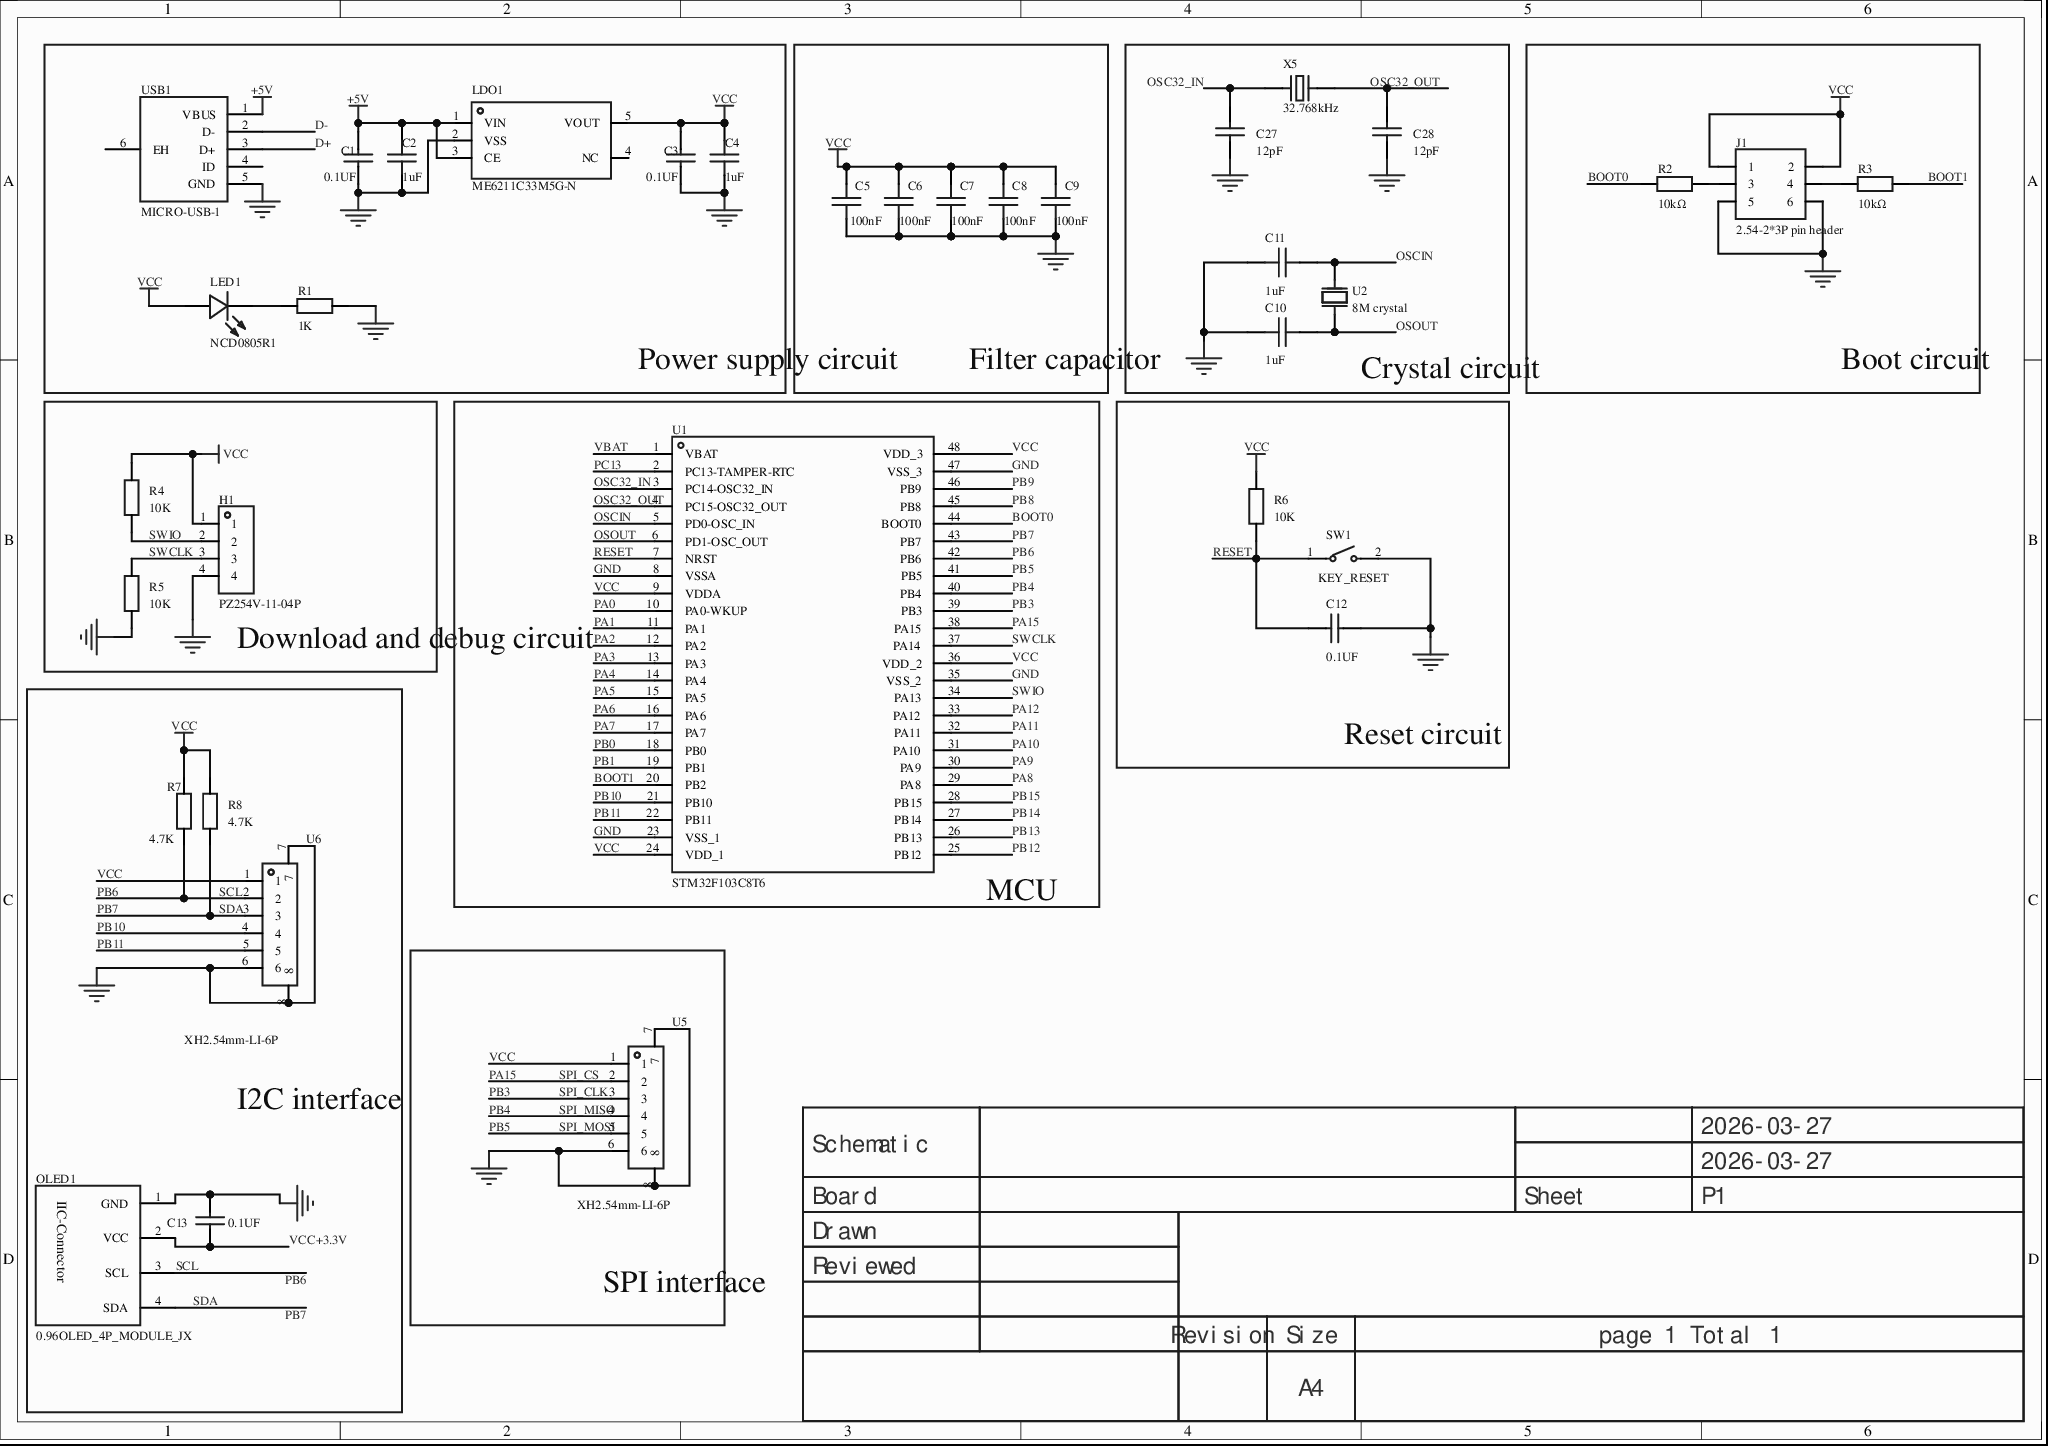
[diagram p0: MISC62287-3.schdoc]
# Altium project MISC62287-2.PrjPcb
1 sheet, 35 parts. Net scope: global (net labels, ports and power ports of the same name join across sheets).
Board file: MISC62287.pcbdoc

## Sheet MISC62287-3.schdoc
size 297 x 209 mm; Version: V1.0; @Project Name: MISC62287; @Update Date: 2026-03-27; @Create Date: 2026-03-27; @Board Name: MISC62287; @Create Time: 22:33:02; @Page Count: 1; @Page No: 1; @Schematic Name: MISC62287; @Update Time: 22:33:02; Size: A4

### Parts
C1  0.1UF  [C0603]
C2  1uF  [C0603]
C3  0.1UF  [C0603]
C4  1uF  [C0603]
C5  100nF  [C0603]
C6  100nF  [C0603]
C7  100nF  [C0603]
C8  100nF  [C0603]
C9  100nF  [C0603]
C10  1uF  [C0603]
C11  1uF  [C0603]
C12  0.1UF  [C0603]
C13  0.1UF  [C0603]
C27  12pF  [R0402]
C28  12pF  [R0402]
H1  PZ254V-11-04P  [HDR-TH_4P-P2.54-V-M]
J1  2.54-2*3P pin header  [HDR-TH_6P-P2.54-V-M-R2-C3-S2.54-1]
LDO1  ME6211C33M5G-N  [SOT-23-5_L3.0-W1.7-P0.95-LS2.8-BL]
LED1  NCD0805R1  [LED0805-RD]
OLED1  0.96OLED_4P_MODULE_JX  [0.96OLED_4P]
R1  1K  [R0603]
R2  10kΩ  [R0603]
R3  10kΩ  [R0603]
R4  10K  [R0603]
R5  10K  [R0603]
R6  10K  [R0603]
R7  4.7K  [R0603]
R8  4.7K  [R0603]
SW1  KEY_RESET  [SW-SMD_L6.0-W3.3-LS8.0]
U1  STM32F103C8T6  [LQFP-48_L7.0-W7.0-P0.50-LS9.0-BL]
U2  8M crystal  [HC-49S_L11.5-W4.7-P4.88]
U5  XH2.54mm-LI-6P  [CONN-SMD_6P-P2.50-H]
U6  XH2.54mm-LI-6P  [CONN-SMD_6P-P2.50-H]
USB1  MICRO-USB-1  [MICRO-USB-SMD_C9900008946]
X5  32.768kHz  [OSC-SMD_L3.2-W1.5]

### Blocks framed on the sheet
Power supply circuit: C1-C4 LDO1 LED1 R1 USB1
Filter capacitor: C5-C9
Crystal circuit: C10 C11 C27 C28 U2 X5
Boot circuit: J1 R2 R3
Download and debug circuit: H1 R4 R5
MCU: U1
Reset circuit: C12 R6 SW1
I2C interface: C13 OLED1 R7 R8 U6
SPI interface: U5

### Nets
+5V: C1.2 C2.2 LDO1.1(VIN) LDO1.3(CE) USB1.1(VBUS)
GND: C1.1 C2.1 C3.1 C4.1 C5.1 C6.1 C7.1 C8.1 C9.1 C10.2 C11.2 C12.1 C13.2 C27.1 C28.1 H1.4 J1.5 J1.6 LDO1.2(VSS) OLED1.1(GND) R1.2 R5.1 SW1.2 U1.8(VSSA) U1.23(VSS_1) U1.35(VSS_2) U1.47(VSS_3) U5.6 U5.7 U5.8 U6.6 U6.7 U6.8 USB1.5(GND)
VCC: C3.2 C4.2 C5.2 C6.2 C7.2 C8.2 C9.2 H1.1 J1.1 J1.2 LDO1.5(VOUT) LED1.2(+) R4.2 R6.2 R7.2 R8.2 U1.9(VDDA) U1.24(VDD_1) U1.36(VDD_2) U1.48(VDD_3) U5.1 U6.1
BOOT0: R2.1 U1.44(BOOT0)
BOOT1: R3.2 U1.20(PB2)
D+: USB1.3(D+)
D-: USB1.2(D-)
OSC32_IN: C27.2 U1.3(PC14-OSC32_IN) X5.1
OSC32_OUT: C28.2 U1.4(PC15-OSC32_OUT) X5.2
OSCIN: C11.1 U1.5(PD0-OSC_IN) U2.1(OSC1)
OSOUT: C10.1 U1.6(PD1-OSC_OUT) U2.2(OSC2)
PA0: U1.10(PA0-WKUP)
PA1: U1.11(PA1)
PA2: U1.12(PA2)
PA3: U1.13(PA3)
PA4: U1.14(PA4)
PA5: U1.15(PA5)
PA6: U1.16(PA6)
PA7: U1.17(PA7)
PA8: U1.29(PA8)
PA9: U1.30(PA9)
PA10: U1.31(PA10)
PA11: U1.32(PA11)
PA12: U1.33(PA12)
PA15: U1.38(PA15) U5.2  [also labelled SPI_CS]
PB0: U1.18(PB0)
PB1: U1.19(PB1)
PB3: U1.39(PB3) U5.3  [also labelled SPI_CLK]
PB4: U1.40(PB4) U5.4  [also labelled SPI_MISO]
PB5: U1.41(PB5) U5.5  [also labelled SPI_MOSI]
PB6: OLED1.3(SCL) R7.1 U1.42(PB6) U6.2  [also labelled SCL]
PB7: OLED1.4(SDA) R8.1 U1.43(PB7) U6.3  [also labelled SDA]
PB8: U1.45(PB8)
PB9: U1.46(PB9)
PB10: U1.21(PB10) U6.4
PB11: U1.22(PB11) U6.5
PB12: U1.25(PB12)
PB13: U1.26(PB13)
PB14: U1.27(PB14)
PB15: U1.28(PB15)
PC13: U1.2(PC13-TAMPER-RTC)
RESET: C12.2 R6.1 SW1.1 U1.7(NRST)
SWCLK: H1.3 R5.2 U1.37(PA14)
SWIO: H1.2 R4.1 U1.34(PA13)
VBAT: U1.1(VBAT)
VCC+3.3V: C13.1 OLED1.2(VCC)
NetJ1_3: J1.3 R2.2
NetJ1_4: J1.4 R3.1
NetLED1_1: LED1.1(-) R1.1

Not connected (* = marked no-connect by the designer): LDO1 4(NC)*; USB1 4(ID)* 6(EH)*

### Notes on the sheet
- 2026-03-27
- Schematic
- Board
- Sheet
- P1
- Drawn
- Reviewed
- Revision
- Size
- A4
- page 1 Total 1

### Library data of the parts
C1 C3 C12 = CAPCER0.1UF16VX5R0603,CAPCER0.1UF25VX5R0603,CAPCER0.1UF16VX7R0603: AddInBom: yes; ModelId: ac125912035d415993ca9572d50418b10819f05c4eef4c71ace90d822a990e87; ModelName: C0603_L1.6-W0.8-H0.8; ModelTransform: 62.992,31.496,0,0,0,0,0,0,0; Symbol: CAPCER0.1UF16VX5R0603,CAPCER0.1UF25VX5R0603,CAPCER0.1UF16VX7R0603; Device: CAPCER0.1UF16VX5R0603,CAPCER0.1UF25VX5R0603,CAPCER0.1UF16VX7R0603; Manufacturer Part: 0.1UF; LCSC Part Name: CAPCER0.1UF16VX5R0603,CAPCER0.1UF25VX5R0603,CAPCER0.1UF16VX7R0603; SupplierPart: C9900012833; Supplier Footprint: C0603; JLCPCB Part Class: Extended Part; Supplier: LCSC; ConvertToPcb: yes; FootprintName: C0603
C2 C4 C10 C11 = CL10A105KB8NNNC: Capacitance:1uF;Tolerance:±10%;Rated voltage:50V;Temperature coefficient:X5R;; Manufacturer: SAMSUNG(三星); AddInBom: yes; ModelId: ac125912035d415993ca9572d50418b10819f05c4eef4c71ace90d822a990e87; ModelName: C0603_L1.6-W0.8-H0.8; ModelTransform: 62.992,31.496,0,0,0,0,0,0,0; Tolerance: ±10%; Voltage Rating: 50V; Temperature Coefficient: X5R; Symbol: CL10A105KB8NNNC; Device: CL10A105KB8NNNC; LCSC Part Name: 1uF ±10% 50V; SupplierPart: C15849; ManufacturerPart: CL10A105KB8NNNC; Supplier Footprint: 0603; JLCPCB Part Class: Basic Part; Datasheet: https://example.com/datasheet/16531.html; Supplier: LCSC; ConvertToPcb: yes; FootprintName: C0603; Value: 1uF
C5-C9 = CC0603KPX7R7BB104: Capacitance:100nF;Tolerance:±10%;Rated voltage:16V;Temperature coefficient:X7R;; Manufacturer: YAGEO(国巨); AddInBom: yes; ModelId: ac125912035d415993ca9572d50418b10819f05c4eef4c71ace90d822a990e87; ModelName: C0603_L1.6-W0.8-H0.8; ModelTransform: 62.992,31.496,0,0,0,0,0,0,0; Tolerance: ±10%; Voltage Rating: 16V; Temperature Coefficient: X7R; Symbol: CC0603KPX7R7BB104; Device: CC0603KPX7R7BB104; LCSC Part Name: 100nF ±10% 16V; SupplierPart: C2649559; ManufacturerPart: CC0603KPX7R7BB104; Supplier Footprint: 0603; JLCPCB Part Class: Extended Part; Datasheet: https://example.com/datasheet/2741468.html; Supplier: LCSC; ConvertToPcb: yes; FootprintName: C0603; Value: 100nF
C13 = CAPCER0.1UF16VX5R0603,CAPCER0.1UF25VX5R0603,CAPCER0.1UF16VX7R0603: 3D Model: ac125912035d415993ca9572d50418b10819f05c4eef4c71ace90d822a990e87; 3D Model Transform: 62.992,31.496,0,0,0,0,0,0,0; AddInBom: yes; ModelName: C0603_L1.6-W0.8-H0.8; Symbol: CAPCER0.1UF16VX5R0603,CAPCER0.1UF25VX5R0603,CAPCER0.1UF16VX7R0603; Device: CAPCER0.1UF16VX5R0603,CAPCER0.1UF25VX5R0603,CAPCER0.1UF16VX7R0603; Manufacturer Part: 0.1UF; LCSC Part Name: CAPCER0.1UF16VX5R0603,CAPCER0.1UF25VX5R0603,CAPCER0.1UF16VX7R0603; Supplier Part: C9900012833; Supplier Footprint: C0603; JLCPCB Part Class: Extended Part; Supplier: LCSC; ConvertToPcb: yes; FootprintName: C0603
C27 C28 = 0402CG120J500NT: Capacitance:12pF;Tolerance:±5%;Rated voltage:50V;Material (temperature coefficient):C0G;; Manufacturer: FH(风华); 3D Model: 36a51122f27c49738f86b3bfa98863e0; 3D Model Transform: 39.37,19.685,0,0,0,0,0,0,0; Tolerance: ±5%; Voltage Rated: 50V; Temperature Coefficient: C0G; AddInBom: yes; ModelName: C0402_L1.0-W0.5-H0.5; Symbol: 0402CG120J500NT; Device: 0402CG120J500NT; Value: 12pF; LCSC Part Name: 12pF ±5% 50V; Supplier Part: C1547; Manufacturer Part: 0402CG120J500NT; Supplier Footprint: 0402; JLCPCB Part Class: Basic library; Datasheet: https://example.com/pdf/20200305/C486355_26A10D38EF8C2A5C37091D0039909270.pdf; Supplier: LCSC; ConvertToPcb: yes; FootprintName: R0402
H1 = PZ254V-11-04P: Pin structure:1x4P;Pitch:2.54mm;Row spacing:-;Round/square pin:Square;Mounting:Through-hole;Rows:Single row;Total pin count:4P;Rated current:3A;Rated voltage:250V;Mating pin length:6mm;Plastic height:2.5mm;Terminal pin length:3mm;Contact material:-;Operating temperature:-40℃~+105℃;Color:Black;; Manufacturer: XFCN(兴飞); Symbol: PZ254V-11-04P_C2691448; AddInBom: yes; ModelId: 112f4d05e8d64e99ab9a333894bea4f90819f05c4eef4c71ace90d822a990e87; ModelName: HDR-TH_4P-P2.54-M-LI-1X4P; ModelTransform: 399.999,104.7242,0,0,0,0,0,0,-118.11; Pin Structure: 1x4P; Pitch: 2.54mm; Circluar Pins/Square Pins: Square; Current Rating: 3A; Voltage Rating (Max): 250V; Device: PZ254V-11-04P; LCSC Part Name: 1x4P 间距:2.54mm 方针 直插; SupplierPart: C2691448; ManufacturerPart: PZ254V-11-04P; Supplier Footprint: 插件,P=2.54mm; JLCPCB Part Class: Extended Part; Datasheet: https://example.com/datasheet/PZ254V-11-04P/2801085.html; Supplier: LCSC; ConvertToPcb: yes; FootprintName: HDR-TH_4P-P2.54-V-M; Row Spacing: -; Mounting Type: Through-hole; Number of Rows: Single row; Number of Pins: 4P; Length of Mating Pin: 6mm; Insulation Height: 2.5mm; Length of End Connection Pin: 3mm; Contact Material: -; Operating Temperature: -40℃~+105℃; Color: Black
J1 = 2.54-2*3P针: Pin structure:-;Pitch:2.54mm;Row spacing:2.54mm;Round/square pin:-;Mounting:Through-hole;Rows:Dual row;Total pin count:6P;Rated current:-;Rated voltage:-;Mating pin length:-;Plastic height:-;Contact material:-;Contact plating:-;Color:Black;; Manufacturer: BOOMELE(博穆精密); Symbol: Header-Male-2.54_2x3; AddInBom: yes; ModelId: fd1b55b786fb415ca65c4187088147b70819f05c4eef4c71ace90d822a990e87; ModelName: HDR2.54-M-LI-2x3P; ModelTransform: 299.9994,200,0,0,0,0,0,0,-118.11; Pitch: 2.54mm; Device: 2.54-2*3P pin header; LCSC Part Name: 间距:2.54mm 直插; SupplierPart: C65114; ManufacturerPart: 2.54-2*3P针; Supplier Footprint: 插件,P=2.54mm; JLCPCB Part Class: Extended Part; Supplier: LCSC; ConvertToPcb: yes; FootprintName: HDR-TH_6P-P2.54-V-M-R2-C3-S2.54-1; Pin Structure: -; Row Spacing: 2.54mm; Circluar Pins/Square Pins: -; Mounting Type: Through-hole; Number of Rows: Dual row; Number of Pins: 6P; Current Rating: -; Voltage Rating (Max): -; Length of Mating Pin: -; Insulation Height: -; Contact Material: -; Contact Plating: -; Color: Black
LDO1 = ME6211C33M5G-N: Output type:Fixed;Operating voltage:6V;Output voltage:3.3V;Output current:500mA;PSRR:70dB@(1kHz);Output polarity:Positive;; Manufacturer: MICRONE(南京微盟); AddInBom: yes; ModelId: 0a2a1b8f50944f73965918ad6e5fe1670819f05c4eef4c71ace90d822a990e87; ModelName: SOT-23-5_L2.9-W1.6-H1.1-LS2.8-P0.95; ModelTransform: 118.60433,114.173,0,90,0,0,0.0005,0.0005,0; Output Type: Fixed; Voltage - Supply: 6V; Output Voltage: 3.3V; Output Current: 500mA; Voltage Dropout: 120mV@(100mA); standby current: 60uA; Noise: 50uVrms; Number of Outputs: 1; Symbol: ME6211C33M5G-N; Device: ME6211C33M5G-N; LCSC Part Name: 输入6V 输出3.3V 500mA; SupplierPart: C82942; ManufacturerPart: ME6211C33M5G-N; Supplier Footprint: SOT-23-5; JLCPCB Part Class: Extended Part; Datasheet: https://example.com/datasheet/84106.html; Supplier: LCSC; ConvertToPcb: yes; FootprintName: SOT-23-5_L3.0-W1.7-P0.95-LS2.8-BL; Power Supply Rejection Ratio (PSRR): 70dB@(1kHz); Features: Overcurrent protection; enable; short-circuit protection; Operating Temperature: -40℃~+150℃; Output Configuration: Positive
LED1 = NCD0805R1: Lamp head type:-;Emission color:Red;Forward voltage drop (Vf):1.6V~2.6V;Power:65mW;Forward current:25mA;Wavelength:615nm~630nm;Diode configuration:Discrete diode;Lens color:-;Color temperature:-;Luminous intensity:195mcd;Viewing angle:130°;Packaging:-;Operating temperature:-30℃~+85℃;; Manufacturer: 国星光电; Symbol: FC-2012HRK-620D; AddInBom: yes; ModelId: b1c5ed7a4f6e46d3bc6f6cc7c20f3fea0819f05c4eef4c71ace90d822a990e87; ModelTransform: 79.527,49.2125,0,0,0,0,0,0,0; Illumination Color: Red; Power(Watts): 65mW; Forward Current: 25mA; Peak Wavelength: 630nm; Luminous Intensity: 195mcd; Viewing Angle: 130°; Device: NCD0805R1; LCSC Part Name: 片式发光二极管; SupplierPart: C84256; ManufacturerPart: NCD0805R1; Supplier Footprint: 0805; JLCPCB Part Class: Basic Part; Datasheet: https://example.com/datasheet/85425.html; Supplier: LCSC; ConvertToPcb: yes; FootprintName: LED0805-RD; ModelName: LED0805-RD; Lamp Holder Type: -; Voltage - Forward(Vf): 1.6V~2.6V; Wavelength - Dominant: 615nm~630nm; Diode Configuration: Discrete diode; Lens Color: -; Color Temperature: -; Mounting Style: -; Operating Temperature: -30℃~+85℃
OLED1 = 0.96OLED_4P_MODULE_JX: AddInBom: yes; ModelId: 79c000fdb68d45a296c2e9bedf4f90550819f05c4eef4c71ace90d822a990e87; ModelTransform: 1393.69792,1318.895,0,0,0,0,0,-560.079,-137.795; Symbol: 0.96OLED_4P_MODULE_JX; Device: 0.96OLED_4P_MODULE_JX; LCSC Part Name: 0.96OLED_4P_MODULE_JX; SupplierPart: C9900004566; ManufacturerPart: 0.96OLED_4P_MODULE_JX; Supplier Footprint: 插件; JLCPCB Part Class: Extended Part; Supplier: LCSC; ConvertToPcb: yes; FootprintName: 0.96OLED_4P; ModelName: 0.96OLED_4P
R1 R4-R8 = Res_0603: Symbol: Resistor; ConvertToPcb: yes; ModelId: fc143cca1e79419f9cd78b61e9279f080819f05c4eef4c71ace90d822a990e87; ModelTransform: 31.8897,63.7794,0,90,0,0,0,0,0; Device: Res_0603; AddInBom: yes; Supplier Footprint: 0603; FootprintName: R0603; ModelName: R0603
  R1: Value: 1K
  R4-R6: Value: 10K
  R7 R8: Value: 4.7K
R2 R3 = 0603WAF1002T5E: Resistor type:Thick-film resistor;Resistance:10kΩ;Tolerance:±1%;Power:100mW;Operating voltage:75V;Temperature coefficient:±100ppm/℃;; Manufacturer: UNI-ROYAL(厚声); AddInBom: yes; ModelId: fc143cca1e79419f9cd78b61e9279f080819f05c4eef4c71ace90d822a990e87; ModelTransform: 31.8897,63.7794,0,90,0,0,0,0,0; Tolerance: ±1%; Power(Watts): 100mW; Voltage-Supply(Max): 75V; Symbol: 0603WAF1002T5E; Device: 0603WAF1002T5E; LCSC Part Name: 厚膜电阻 10kΩ ±1% 100mW; SupplierPart: C25804; ManufacturerPart: 0603WAF1002T5E; Supplier Footprint: 0603; JLCPCB Part Class: Basic Part; Datasheet: https://example.com/datasheet/26547.html; Supplier: LCSC; ConvertToPcb: yes; FootprintName: R0603; ModelName: R0603; Type: Thick-film resistor; Value: 10kΩ; Temperature Coefficient: ±100ppm/℃; Operating Temperature: -55℃~+155℃
SW1 = SW_PB2_A1: AddInBom: yes; ModelId: b2f4ea9f0afc4b0786d53dba66ceb9e40819f05c4eef4c71ace90d822a990e87; ModelName: SW-SMD_L6.0-W3.3-H5-LS8.0; ModelTransform: 314.96,129.921,0,0,0,0,0,0,0; Symbol: SW_PB2_A1; Device: SW_PB2_A1; Manufacturer Part: KEY_RESET; LCSC Part Name: SW_PB2_A1; SupplierPart: C9900015236; Supplier Footprint: SW_3*6*2.5mm; JLCPCB Part Class: Extended Part; Supplier: LCSC; ConvertToPcb: yes; FootprintName: SW-SMD_L6.0-W3.3-LS8.0
U1 = STM32F103C8T6: CPU core:ARM-M3;Max CPU frequency:72MHz;Application field:-;; Manufacturer: ST(意法半导体); AddInBom: yes; ModelId: 093be70396ff421eb2cdb946d5311efc0819f05c4eef4c71ace90d822a990e87; ModelName: LQFP-48_L7.0-W7.0-H1.4-LS9.0-P0.50; ModelTransform: 354.331,354.331,0,0,0,0,0,0,0; CPU Core: ARM-M3; CPU Maximum Speed: 72MHz; Program Storage Size: 64KB; Program Memory Type: FLASH; Number of I/O: 37; ADC (Bit): 12bit; Voltage - Supply: 2V~3.6V; Symbol: STM32F103C8T6; Device: STM32F103C8T6; LCSC Part Name: 主流增强型ARM Cortex-M3 MCU，具有64 KB Flash、72 MHz CPU、电机控制、USB和CAN; SupplierPart: C8734; ManufacturerPart: STM32F103C8T6; Supplier Footprint: LQFP-48(7x7); JLCPCB Part Class: Extended Part; Datasheet: https://example.com/datasheet/9243.html; Supplier: LCSC; ConvertToPcb: yes; FootprintName: LQFP-48_L7.0-W7.0-P0.50-LS9.0-BL; Applications: -
U2 = 8M晶振_C9900011272: ManufacturerPart: 8M晶振; Device: 8M crystal_C9900011272; AddInBom: yes; ModelId: 8681f9edbc4c49baa7439b9863851e5c0819f05c4eef4c71ace90d822a990e87; ModelTransform: 452.755,183.4642,0,0,0,0,0,0,-137.795; Symbol: 8M crystal; LCSC Part Name: 8M晶振; SupplierPart: C9900011272; Supplier Footprint: HC-49S; JLCPCB Part Class: Extended Part; Supplier: LCSC; ConvertToPcb: yes; FootprintName: HC-49S_L11.5-W4.7-P4.88; ModelName: HC-49S_L11.5-W4.7-P4.88
U5 U6 = XH2.54mm-LI-6P: AddInBom: yes; ModelId: d00e98fc2787443b99850c08410b29640819f05c4eef4c71ace90d822a990e87; ModelTransform: 787.4,401.574,0,0,0,0,0,-6.89,0; Symbol: XH2.54MM-LI-6P; Device: XH2.54mm-LI-6P; LCSC Part Name: XH2.54mm-LI-6P; SupplierPart: C2842318; ManufacturerPart: XH2.54mm-LI-6P; Supplier Footprint: SMD-6_7.8X17.5X2.5P; JLCPCB Part Class: Extended Part; Supplier: LCSC; ConvertToPcb: yes; FootprintName: CONN-SMD_6P-P2.50-H; ModelName: CONN-SMD_6P-P2.50-H
USB1 = MICRO-USB-1: AddInBom: yes; ModelId: 03278485a0ad4b6f9ea4a64b4dabf4cb0819f05c4eef4c71ace90d822a990e87; ModelTransform: 314.96,223.6216,0,0,0,0,0,-49.213,-39.37; Symbol: MICRO-USB-1; Device: MICRO-USB-1; LCSC Part Name: MICRO-USB-1; SupplierPart: C9900008946; ManufacturerPart: MICRO-USB-1; Supplier Footprint: USB-micro; JLCPCB Part Class: Extended Part; Supplier: LCSC; ConvertToPcb: yes; FootprintName: MICRO-USB-SMD_C9900008946; ModelName: MICRO-USB-SMD_C9900008946
X5 = X321532768KGD2SI: Crystal type:SMD crystal;Frequency:32.768kHz;Frequency deviation at room temp:±20ppm;External load capacitance:12.5pF;Frequency stability (full temp):-;; Manufacturer: YXC(扬兴晶振); 3D Model: 2dd241c0893b4675b8def6f6998a8251; 3D Model Transform: 125.984,59.055,0,0,0,0,0,-0.0005,0; Normal temperature Frequency Tolerance: ±20ppm; External load capacitor: 12.5pF; AddInBom: yes; ModelName: OSC-SMD_L3.2-W1.5-H0.8; Symbol: X321532768KGD2SI; Device: X321532768KGD2SI; Value: 32.768kHz; LCSC Part Name: 32.768kHz ±20ppm 12.5pF; Supplier Part: C620155; Manufacturer Part: X321532768KGD2SI; Supplier Footprint: SMD3215-2P; JLCPCB Part Class: Extended library; Datasheet: https://example.com/pdf/20240329/3A7650FD985DD0DE85694D3785AB4916.pdf; Supplier: LCSC; Crystal Type: SMD crystal; Frequency Stability(Full temperature range): -; Operating Temperature: -40℃~+85℃; ConvertToPcb: yes; FootprintName: OSC-SMD_L3.2-W1.5